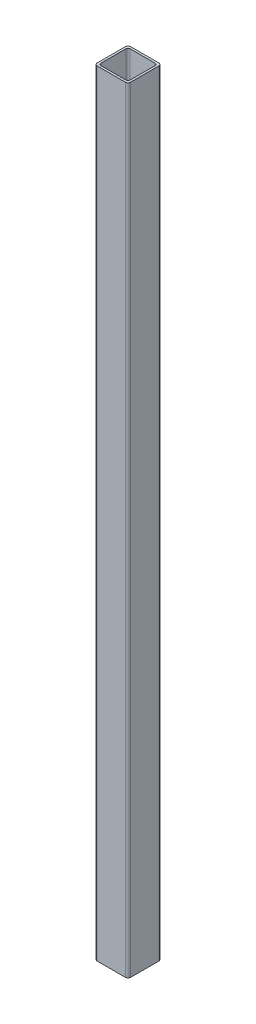
SolidWorks part; units mm, degrees
material "Angle steel 100×100×6/Q235"
ref_plane "Front Plane" through (0, 0, 0) normal (0, 0, 1) x (1, 0, 0)
ref_plane "Top Plane" through (0, 0, 0) normal (0, 1, 0) x (1, 0, 0)
ref_plane "Right Plane" through (0, 0, 0) normal (1, 0, 0) x (0, 0, -1)
sketch "Sketch2" plane through (0, 0, 0) normal (0, 1, 0) x (1, 0, 0)
  line L0 (12.6, 4.775) -> (87.4, 4.775)
  line L1 (6.3, 11.075) -> (6.3, 85.875)
  line L2 (87.4, 92.175) -> (12.6, 92.175)
  line L3 (93.7, 85.875) -> (93.7, 11.075)
  line L4 (7.875, -1.525) -> (92.125, -1.525)
  line L5 (0, 6.35) -> (0, 90.6)
  line L6 (92.125, 98.475) -> (7.875, 98.475)
  line L7 (100, 90.6) -> (100, 6.35)
  arc A0 (100, 90.6) -> (92.125, 98.475) centre (92.125, 90.6) ccw
  arc A1 (92.125, -1.525) -> (100, 6.35) centre (92.125, 6.35) ccw
  arc A2 (0, 6.35) -> (7.875, -1.525) centre (7.875, 6.35) ccw
  arc A3 (7.875, 98.475) -> (0, 90.6) centre (7.875, 90.6) ccw
  arc A4 (12.6, 92.175) -> (6.3, 85.875) centre (12.6, 85.875) ccw
  arc A5 (93.7, 85.875) -> (87.4, 92.175) centre (87.4, 85.875) ccw
  arc A6 (87.4, 4.775) -> (93.7, 11.075) centre (87.4, 11.075) ccw
  arc A7 (6.3, 11.075) -> (12.6, 4.775) centre (12.6, 11.075) ccw
extrude "Boss-Extrude1" add sketch "Sketch2" along normal blind 2320
